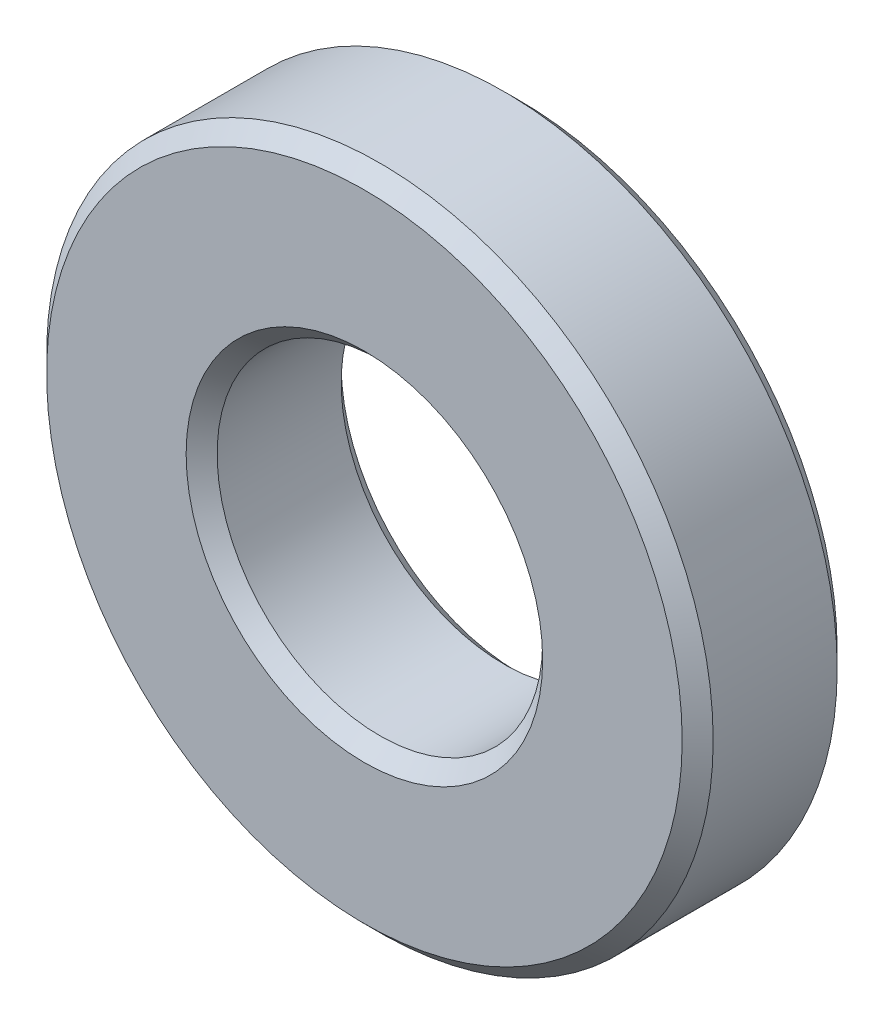
SolidWorks part; units mm, degrees
material "Q235-AF (FL)"
ref_plane "Front Plane" through (0, 0, 0) normal (0, 0, 1) x (1, 0, 0)
ref_plane "Top Plane" through (0, 0, 0) normal (0, 1, 0) x (1, 0, 0)
ref_plane "Right Plane" through (0, 0, 0) normal (1, 0, 0) x (0, 0, -1)
sketch "Sketch1" plane through (0, 0, 0) normal (0, 0, 1) x (1, 0, 0)
  circle A0 centre (0, 0) radius 5.25
  circle A1 centre (0, 0) radius 10.75
  dimension "D1" = 10.5
  dimension "D2" = 21.5
extrude "Boss-Extrude1" add sketch "Sketch1" along normal blind 5
chamfer "Chamfer1" distance 0.5 angle 45 4 edges at (10.75, 0, 0) (5.25, 0, 0) (5.25, 0, 5) (10.75, 0, 5)
